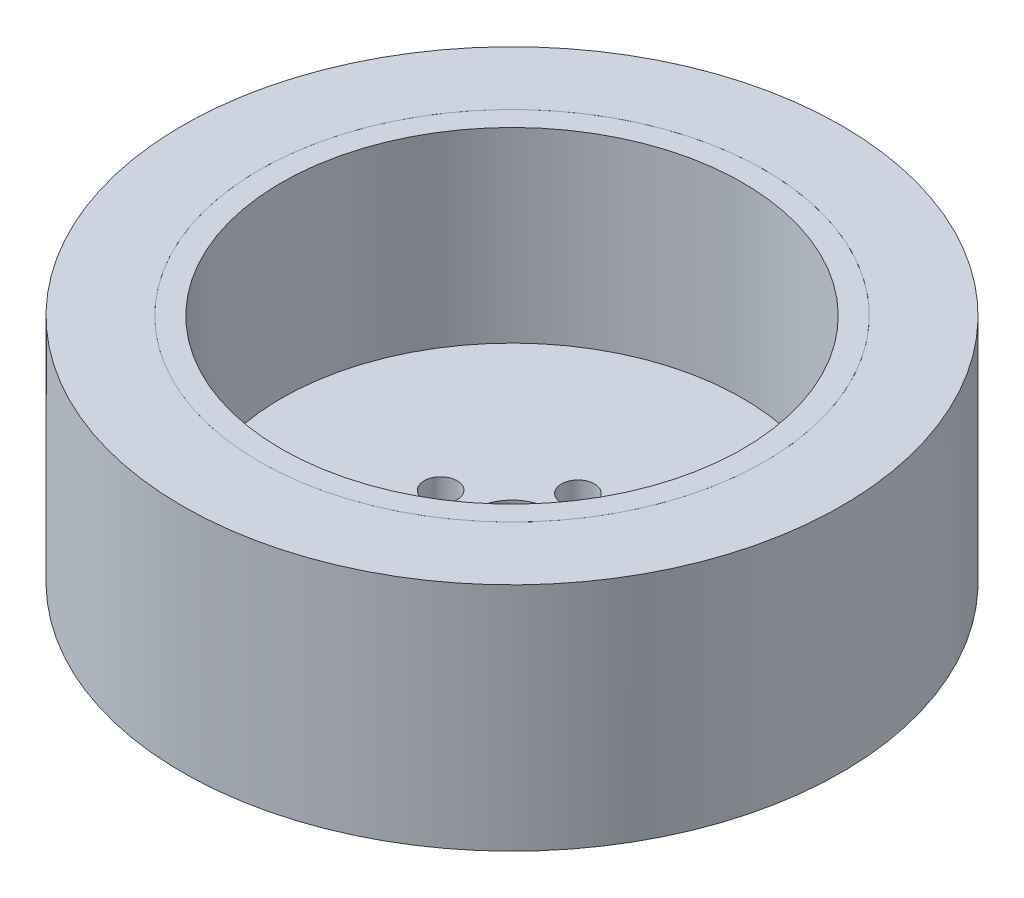
from build123d import *

# Parameters (mm, degrees)
SKETCH1_R           = 23
SKETCH1_R_2         = 1.5
SKETCH1_R_3         = 3.5
BOSS_EXTRUDE1_DEPTH = 4
SKETCH2_R           = 23
SKETCH2_R_2         = 21
BOSS_EXTRUDE2_DEPTH = 17
SKETCH3_R           = 30
SKETCH3_R_2         = 23
BOSS_EXTRUDE3_DEPTH = 21


with BuildPart() as part:
    # Sketch1 → Boss-Extrude1 (new body)
    with BuildSketch(Plane(origin=(0, 0, 0), x_dir=(1, 0, 0), z_dir=(0, 1, 0))):
        with Locations(Location((0, 0, 0), (0, 0, 270))):
            Circle(SKETCH1_R)
        with Locations(Location((6.5, 0, 0), (0, 0, 270))):
            Circle(SKETCH1_R_2, mode=Mode.SUBTRACT)
        with Locations(Location((-6.5, 0, 0), (0, 0, 270))):
            Circle(SKETCH1_R_2, mode=Mode.SUBTRACT)
        with Locations(Location((0, -6, 0), (0, 0, 270))):
            Circle(SKETCH1_R_2, mode=Mode.SUBTRACT)
        with Locations(Location((0, 6, 0), (0, 0, 270))):
            Circle(SKETCH1_R_2, mode=Mode.SUBTRACT)
        with Locations(Location((0, 0, 0), (0, 0, 270))):
            Circle(SKETCH1_R_3, mode=Mode.SUBTRACT)
    extrude(amount=BOSS_EXTRUDE1_DEPTH)

    # Sketch2 → Boss-Extrude2 (add)
    with BuildSketch(Plane(origin=(0, 4, 0), x_dir=(1, 0, 0), z_dir=(0, 1, 0))):
        with Locations(Location((0, 0, 0), (0, 0, 270))):
            Circle(SKETCH2_R)
        with Locations(Location((0, 0, 0), (0, 0, 270))):
            Circle(SKETCH2_R_2, mode=Mode.SUBTRACT)
    extrude(amount=BOSS_EXTRUDE2_DEPTH)


with BuildPart() as body_2:
    # Sketch3 → Boss-Extrude3 (new body)
    with BuildSketch(Plane.XZ):
        with Locations(Location((0, 0, 0), (0, 0, 270))):
            Circle(SKETCH3_R)
        with Locations(Location((0, 0, 0), (0, 0, 270))):
            Circle(SKETCH3_R_2, mode=Mode.SUBTRACT)
    extrude(amount=-BOSS_EXTRUDE3_DEPTH)


solid = Compound([part.part, body_2.part])
